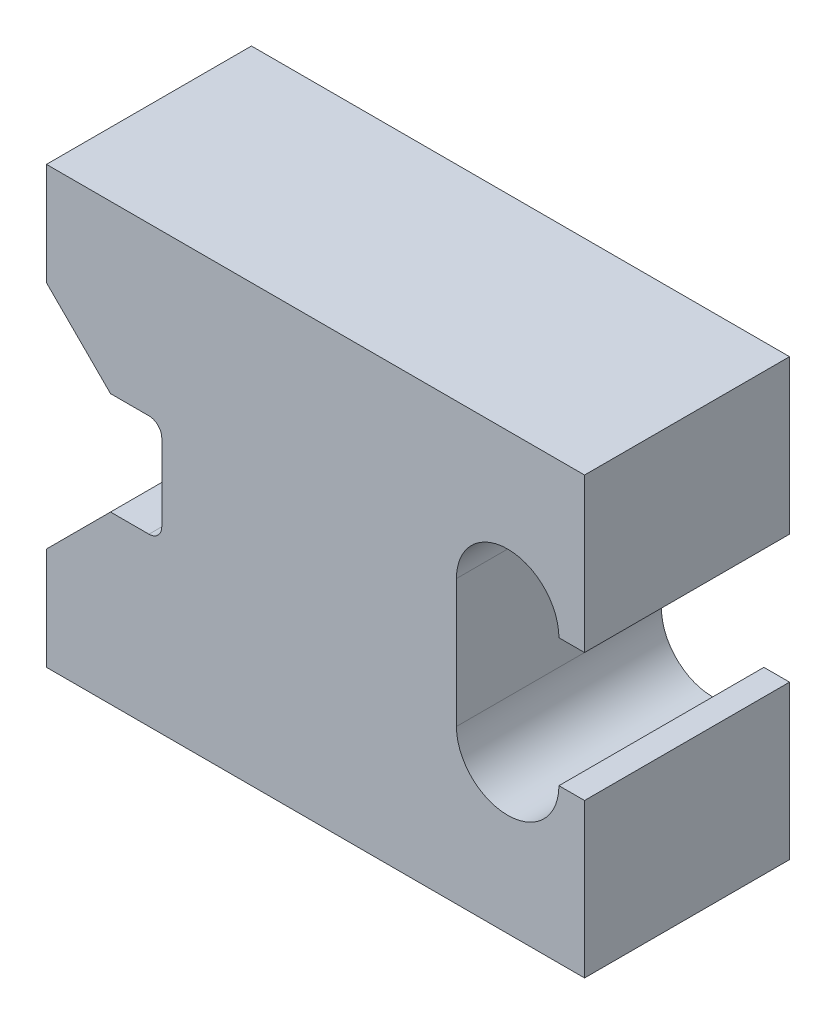
from build123d import *

# Parameters (mm, degrees)
SKETCH1_W          = 45
SKETCH1_H          = 34
BASE_EXTRUDE_DEPTH = 16
CUT_EXTRUDE1_DEPTH = 65.381674411
FILLET1_R          = 1
FILLET2_R          = 1
CUT_EXTRUDE3_DEPTH = 65.381674411
SKETCH5_W          = 3
SKETCH5_H          = 34
CUT_EXTRUDE4_DEPTH = 65.381674411


with BuildPart() as part:
    # Sketch1 → Base-Extrude (new body)
    with BuildSketch(Plane.XY):
        with Locations((37.5, 0)):
            Rectangle(SKETCH1_W, SKETCH1_H)
    extrude(amount=BASE_EXTRUDE_DEPTH)

    # Sketch2 → Cut-Extrude1 (cut, through all)
    with BuildSketch(Plane.XY.offset(16)):
        Polygon((27, 4), (27, -4), (23, -4), (15, -12), (15, 12), (23, 4), align=None)
    extrude(amount=-CUT_EXTRUDE1_DEPTH, mode=Mode.SUBTRACT)

    # Fillet1
    fillet1_edges = [part.edges().sort_by_distance(p)[0] for p in [
        (27, 4, 8),
    ]]
    fillet(fillet1_edges, radius=FILLET1_R)

    # Fillet2
    fillet2_edges = [part.edges().sort_by_distance(p)[0] for p in [
        (27, -4, 8),
    ]]
    fillet(fillet2_edges, radius=FILLET2_R)

    # Sketch4 → Cut-Extrude3 (cut, through all)
    with BuildSketch(Plane.XY.offset(16)):
        with BuildLine():
            Line((50, 5), (50, -5))
            ThreePointArc((50, -5), (54, -9), (58, -5))
            Line((58, -5), (60, -5))
            Line((60, -5), (60, 5))
            Line((60, 5), (58, 5))
            ThreePointArc((58, 5), (54, 9), (50, 5))
        make_face()
    extrude(amount=-CUT_EXTRUDE3_DEPTH, mode=Mode.SUBTRACT)

    # Sketch5 → Cut-Extrude4 (cut, through all)
    with BuildSketch(Plane.XY.offset(16)):
        with Locations((16.5, 0)):
            Rectangle(SKETCH5_W, SKETCH5_H)
    extrude(amount=-CUT_EXTRUDE4_DEPTH, mode=Mode.SUBTRACT)


solid = part.part
